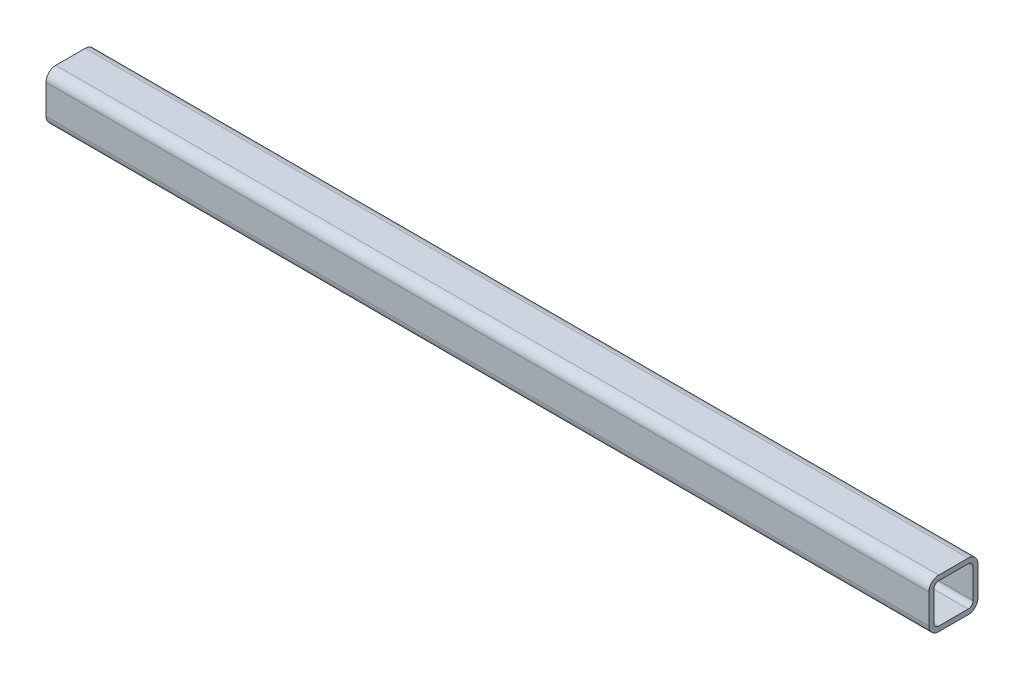
SolidWorks part; units mm, degrees
material "普通碳钢"
ref_plane "Front Plane" through (0, 0, 0) normal (0, 0, 1) x (1, 0, 0)
ref_plane "Top Plane" through (0, 0, 0) normal (0, 1, 0) x (1, 0, 0)
ref_plane "Right Plane" through (0, 0, 0) normal (1, 0, 0) x (0, 0, -1)
sketch "草图1" plane through (0, 0, 0) normal (0, 0, 1) x (1, 0, 0)
  line L0 (-1000, 0) -> (-280, 0)
  dimension "D1" = 720
  dimension "D2" = 1000
other "Square Tube 40 X 40 X 4(1)"
ref_plane "Plane1" through (-1000, 0, 0) normal (1, 0, 0) x (0, 1, 0)
sketch "Sketch1" plane through (-1000, 0, 0) normal (1, 0, 0) x (0, 1, 0)
  line L0 (-12, -16) -> (12, -16)
  line L1 (-16, -12) -> (-16, 12)
  line L2 (12, 16) -> (-12, 16)
  line L3 (16, 12) -> (16, -12)
  line L4 (-12, -20) -> (12, -20)
  line L5 (-20, -12) -> (-20, 12)
  line L6 (12, 20) -> (-12, 20)
  line L7 (20, 12) -> (20, -12)
  arc A0 (20, 12) -> (12, 20) centre (12, 12) ccw
  arc A1 (12, -20) -> (20, -12) centre (12, -12) ccw
  arc A2 (-20, -12) -> (-12, -20) centre (-12, -12) ccw
  arc A3 (-12, 20) -> (-20, 12) centre (-12, 12) ccw
  arc A4 (-12, 16) -> (-16, 12) centre (-12, 12) ccw
  arc A5 (16, 12) -> (12, 16) centre (12, 12) ccw
  arc A6 (12, -16) -> (16, -12) centre (12, -12) ccw
  arc A7 (-16, -12) -> (-12, -16) centre (-12, -12) ccw
  point P0 (-20, 0)
  point P1 (20, 0)
  point P2 (0, 20)
  point P3 (0, -20)
  point P4 (0, 0)
  point P5 (-20, -20)
  point P6 (20, -20)
  point P7 (20, 20)
  point P8 (-20, 20)
  point P33 (0, 0)
  dimension "D1" = 8
  dimension "Thickness" = 4
  dimension "V_leg" = 40
